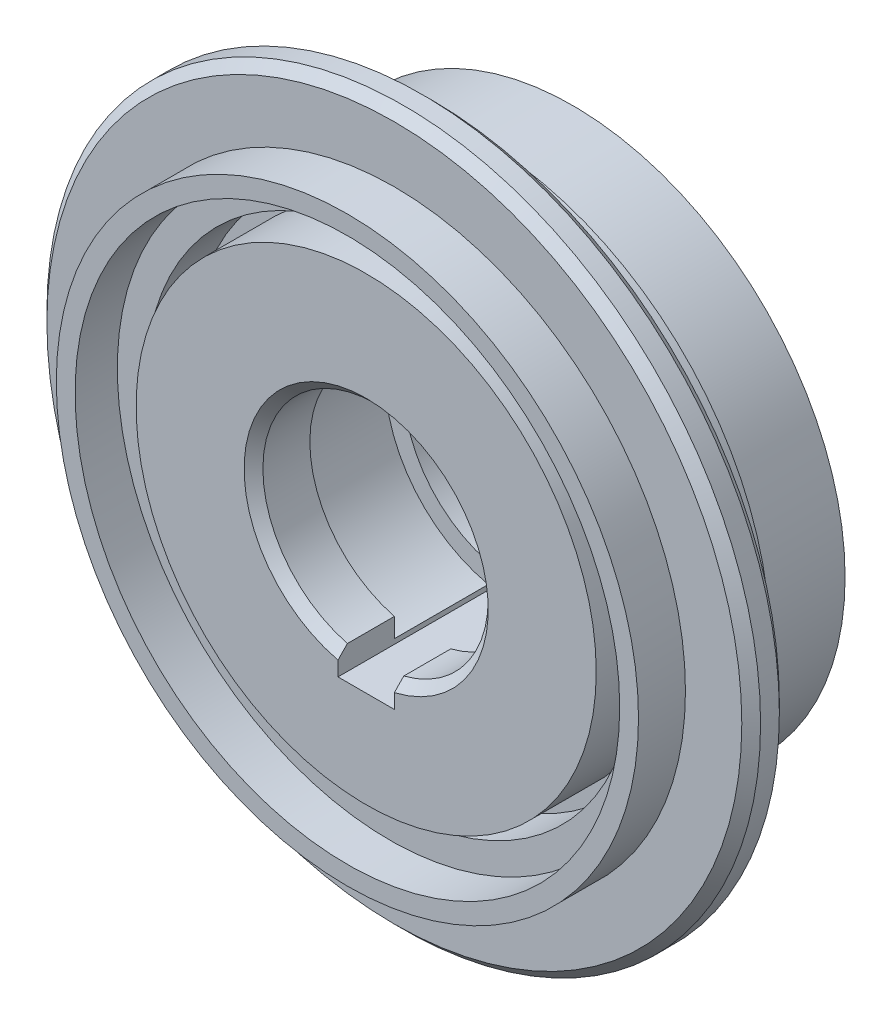
SolidWorks part; units mm, degrees
material "35"
ref_plane "前视基准面" through (0, 0, 0) normal (0, 0, 1) x (1, 0, 0)
ref_plane "上视基准面" through (0, 0, 0) normal (0, 1, 0) x (1, 0, 0)
ref_plane "右视基准面" through (0, 0, 0) normal (1, 0, 0) x (0, 0, -1)
sketch "草图1" plane through (0, 0, 0) normal (0, 1, 0) x (1, 0, 0)
  line L0 (0, 0) -> (0, 31.0262) construction
  line L1 (-12, 22) -> (-12, 16)
  line L2 (-12, 16) -> (-14, 16)
  line L3 (-14, 16) -> (-14, 6)
  line L4 (-14, 6) -> (-12, 6)
  line L5 (-12, 6) -> (-12, 0)
  line L6 (-12, 0) -> (-24.5, 0)
  line L7 (-24.5, 0) -> (-24.5, 7.5)
  line L8 (-24.5, 7.5) -> (-29, 7.5)
  line L9 (-29, 7.5) -> (-29, 22)
  line L10 (-29, 22) -> (-12, 22)
  dimension "D1" = 10
  dimension "D2" = 6
  dimension "D3" = 24
  dimension "D4" = 28
  dimension "D5" = 22
  dimension "D6" = 14.5
  dimension "D7" = 58
  dimension "D8" = 49
revolve "旋转1" add sketch "草图1" angle 360 about L0
sketch "草图2" plane through (0, 0, 0) normal (0, 1, 0) x (1, 0, 0)
  line L0 (-29, 12) -> (-29, 7.5)
  line L1 (-29, 22) -> (-29, 7.5) construction
  line L2 (-29, 7.5) -> (-26, 7.5)
  line L3 (-29, 7.5) -> (29, 7.5) construction
  line L4 (-26, 7.5) -> (-26, 2.5)
  line L5 (-26, 2.5) -> (-29, 2.5)
  line L6 (-29, 2.5) -> (-29, -2)
  line L7 (-29, -2) -> (-31, -2)
  line L8 (-31, -2) -> (-31, 3)
  line L9 (-31, 3) -> (-38, 3)
  line L10 (-38, 3) -> (-38, 7)
  line L11 (-26, 5) -> (-38, 5) construction
  line L12 (29, 22) -> (-29, 22) construction
  line L13 (-24.5, 7.5) -> (-24.5, 0) construction
  line L14 (-29, 12) -> (-31, 12)
  line L15 (-31, 7) -> (-38, 7)
  line L16 (-31, 12) -> (-31, 7)
  line L17 (0, 0) -> (0, 22) construction
  line L18 (12, 22) -> (-12, 22) construction
  dimension "D1" = 17
  dimension "D2" = 24
  dimension "D3" = 4
  dimension "D4" = 1.5
  dimension "D5" = 2
  dimension "D6" = 38
revolve "旋转2" add sketch "草图2" angle 360 about L17
chamfer "倒角1" distance 1 angle 45 2 edges at (38, 0, -3) (38, 0, -7)
sketch "草图3" plane through (0, 0, -22) normal (0, 0, -1) x (-1, 0, 0)
  line L1 (3, -14.2) -> (-3, -14.2)
  line L2 (3, -14.2) -> (3, -9.8)
  line L3 (3, -9.8) -> (-3, -9.8)
  line L4 (-3, -14.2) -> (-3, -9.8)
  line L5 (3, -14.2) -> (-3, -9.8) construction
  line L6 (3, -9.8) -> (-3, -14.2) construction
  circle A0 centre (0, 0) radius 12 construction
  point P0 (0, -12)
  point P7 (0, 0)
  dimension "D1" = 6
  dimension "D2" = 26.2
extrude "切除-拉伸1" cut sketch "草图3" against normal through all
chamfer "倒角2" distance 1 angle 45 2 edges at (0, 12, 0) (0, 12, -22)
